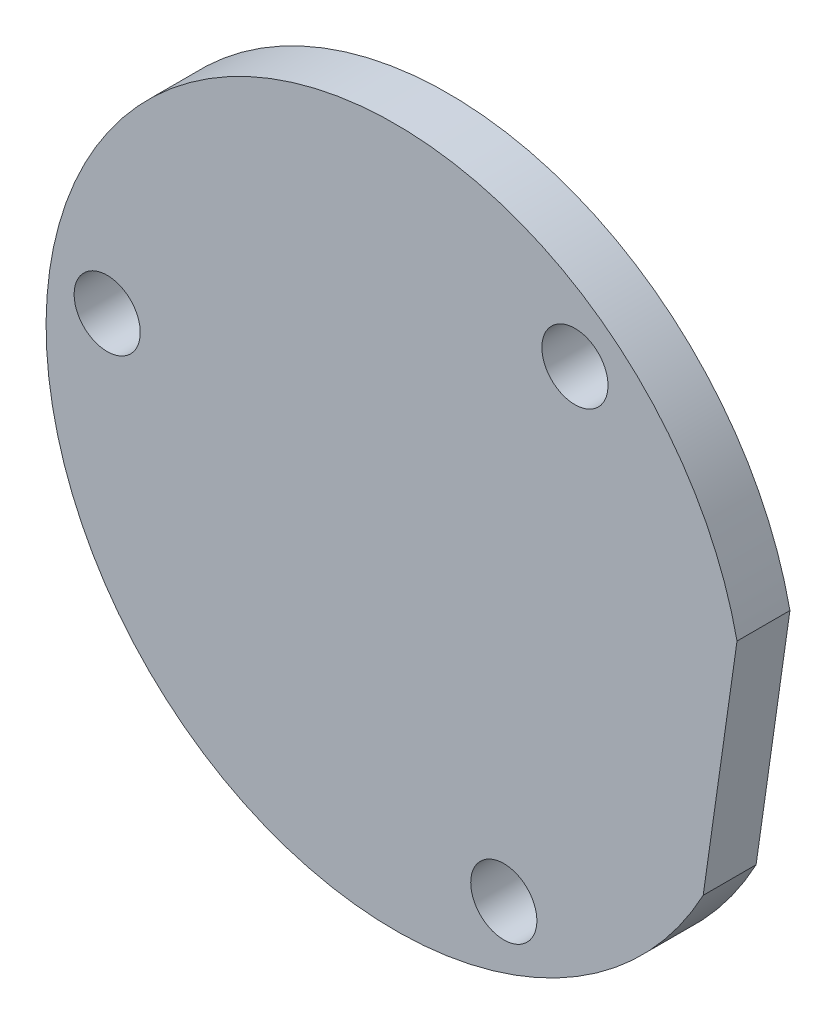
SolidWorks part; units mm, degrees
ref_plane "Front Plane" through (0, 0, 0) normal (0, 0, 1) x (1, 0, 0)
ref_plane "Top Plane" through (0, 0, 0) normal (0, 1, 0) x (1, 0, 0)
ref_plane "Right Plane" through (0, 0, 0) normal (1, 0, 0) x (0, 0, -1)
ref_plane "Plane1" through (0, 0, -144.693) normal (0, 0, 1) x (1, 0, 0)
sketch "Sketch1" plane through (0, 0, -144.693) normal (0, 0, 1) x (1, 0, 0)
  line L0 (511.4594, 9.1231) -> (517.8475, 53.9248)
  arc A0 (517.8475, 53.9248) -> (511.4594, 9.1231) centre (453.2742, 40.2756) ccw
  dimension "D1" = 66
  dimension "D2" = 6.388
  dimension "D3" = 64.5732
extrude "Boss-Extrude1" add sketch "Sketch1" against normal blind 10
ref_plane "Plane2" through (0, 40.2756, 0) normal (0, 1, 0) x (1, 0, 0)
sketch "Sketch2" plane through (0, 40.2756, 0) normal (0, 1, 0) x (1, 0, 0)
  line L0 (498.2742, 158.693) -> (453.2742, 158.693)
  line L1 (453.2742, 158.693) -> (453.2742, 154.693)
  line L2 (453.2742, 154.693) -> (498.2742, 154.693)
  line L3 (498.2742, 154.693) -> (498.2742, 158.693)
  line L4 (453.2742, 158.693) -> (453.2742, 154.693) construction
  dimension "D1" = 45
  dimension "D2" = 4
revolve "Revolve1" add sketch "Sketch2" angle 360 about L4
hole_wizard "Ø12.5 (12.5) Diameter Hole1" positions "Sketch4" profile "Sketch3" hole size "Ø12.5" standard "ANSI Metric"
sketch "Sketch4" plane through (0, 0, -154.693) normal (0, 0, -1) x (-1, 0, 0)
  point P0 (-398.8249, 48.0393)
  point P1 (-487.2224, 83.5483)
  point P2 (-473.7754, -10.7606)
sketch "Sketch3" plane through (398.8249, 48.0393, -154.693) normal (1, 0, 0) x (0, 1, 0)
  line L0 (0, 0) -> (0, 10)
  line L1 (0, 10) -> (6.25, 10)
  line L2 (6.25, 10) -> (6.25, 0)
  line L5 (6.25, 0) -> (0, 0)
  line L11 (0, -6.35) -> (0, 107.95) construction
  dimension "通孔孔直径" = 12.5
  dimension "通孔孔深度" = 10
hole_wizard "M64 Clearance Hole1" positions "Sketch6" profile "Sketch5" hole size "M64" standard "ANSI Metric"
sketch "Sketch6" plane through (0, 0, -158.693) normal (0, 0, -1) x (-1, 0, 0)
  point P0 (-453.2742, 40.2756)
sketch "Sketch5" plane through (453.2742, 40.2756, -158.693) normal (1, 0, 0) x (0, 1, 0)
  line L0 (0, 0) -> (0, 4)
  line L1 (0, 4) -> (35, 4)
  line L2 (35, 4) -> (35, 0)
  line L5 (35, 0) -> (0, 0)
  line L10 (0, 4) -> (-35, 4) construction
  line L11 (0, -6.35) -> (0, 107.95) construction
  dimension "孔直径" = 70
  dimension "孔深度" = 4
  dimension "导头角度" = 180
